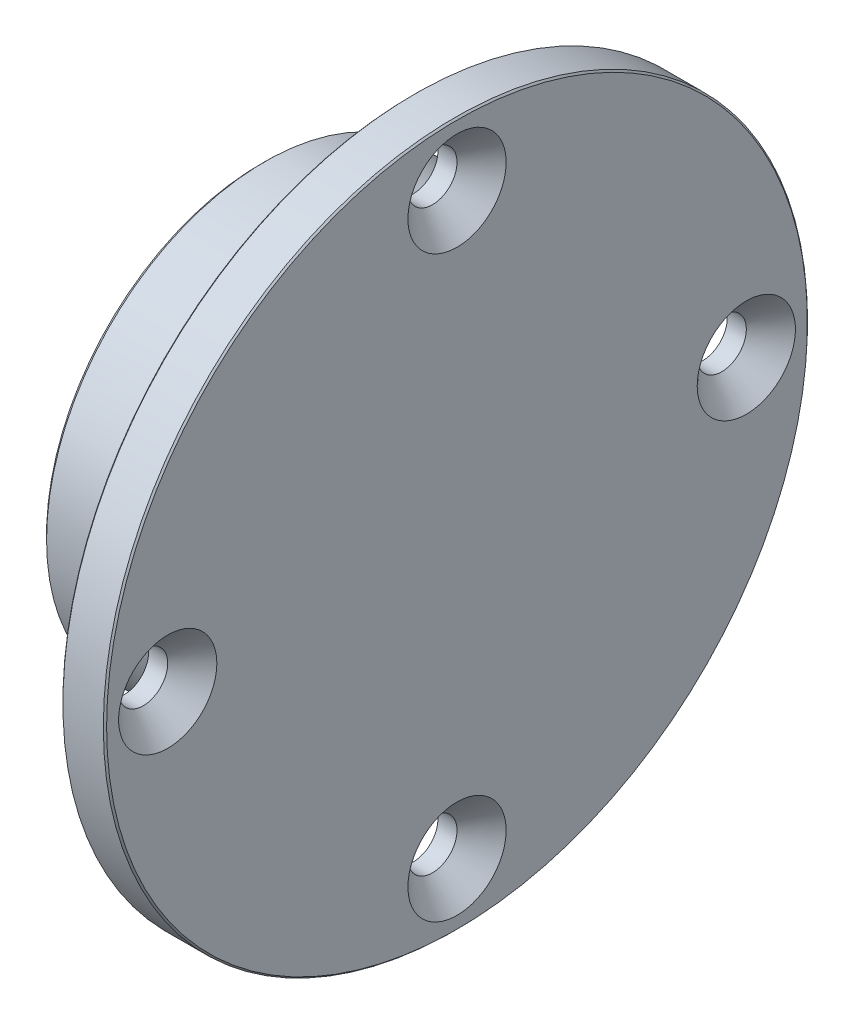
SolidWorks part; units mm, degrees
material "6063-T6"
ref_plane "Front Plane" through (0, 0, 0) normal (0, 0, 1) x (1, 0, 0)
ref_plane "Top Plane" through (0, 0, 0) normal (0, 1, 0) x (1, 0, 0)
ref_plane "Right Plane" through (0, 0, 0) normal (1, 0, 0) x (0, 0, -1)
sketch "Sketch1" plane through (0, 0, 0) normal (0, 0, 1) x (1, 0, 0)
  line L0 (0, 16) -> (1.6954, 16)
  line L1 (13, 16) -> (13, 12.5)
  line L2 (13, 12.5) -> (15, 12.5)
  line L3 (15, 12.5) -> (15, 0)
  line L4 (15, 0) -> (18, 0)
  line L5 (18, 0) -> (18, 32.5)
  line L6 (18, 32.5) -> (14, 32.5)
  line L7 (14, 32.5) -> (14, 20)
  line L8 (14, 20) -> (0, 20)
  line L9 (0, 20) -> (0, 16)
  line L10 (1.6954, 16) -> (1.6954, 16.85)
  line L11 (1.6954, 16.85) -> (2.9954, 16.85)
  line L12 (2.9954, 16.85) -> (2.9954, 16)
  line L13 (2.9954, 16) -> (13, 16)
  dimension "D1" = 16
  dimension "D2" = 2
  dimension "D3" = 12.5
  dimension "D4" = 18
  dimension "D5" = 4
  dimension "D6" = 3
  dimension "D7" = 20
  dimension "D8" = 32.5
  dimension "D9" = 1.3
  dimension "D10" = 16.85
  dimension "D11" = 10.0046
revolve "Revolve1" add sketch "Sketch1" angle 360 about L4
sketch "Sketch2" plane through (0, 0, 0) normal (0, 1, 0) x (1, 0, 0)
  line L0 (14, 26.5) -> (18, 26.5)
  line L1 (14, 32.5) -> (14, -32.5) construction
  line L2 (18, -32.5) -> (18, 32.5) construction
  line L3 (18, 26.5) -> (18, 31)
  line L4 (18, 31) -> (15.75, 28.75)
  line L5 (15.75, 28.75) -> (14, 28.75)
  line L6 (14, 28.75) -> (14, 26.5)
  dimension "D1" = 26.5
  dimension "D2" = 2.25
  dimension "D3" = 4.5
  dimension "D4" = 45
revolve "Cut-Revolve1" cut sketch "Sketch2" angle 360 about L0
pattern_circular "CirPattern1" count 4 over 360 about axis through (0, 0, 0) along (1, 0, 0) of "Cut-Revolve1"
chamfer "Chamfer1" distance 0.4 angle 45 5 edges at (13, 0, 12.5) (0, 0, 16) (18, 0, 32.5) (14, 0, 32.5) (0, 0, 20)
hole_wizard "M4 Tapped Hole1" positions "Sketch4" profile "Sketch5" tap size "M4" standard "GB"
sketch "Sketch4" plane through (18, 0, 0) normal (1, 0, 0) x (0, 0, -1)
  line L0 (0, 0) -> (26.5, 0) construction
  line L2 (0, 0) -> (10.0763, 10.0763) construction
  circle A0 centre (0, 0) radius 14.25
  point P13 (10.0763, 10.0763)
  dimension "D1" = 28.5
  dimension "D2" = 45
cosmetic thread "Hole thread1" [suppressed] parameters "D2"=4
sketch "Sketch5" plane through (18, 10.0763, -10.0763) normal (0, 1, 0) x (0, 0, -1)
  line L0 (0, 0) -> (0, 18)
  line L1 (0, 18) -> (1.65, 18)
  line L2 (1.65, 18) -> (1.65, 0)
  line L5 (1.65, 0) -> (0, 0)
  line L11 (0, -6.35) -> (0, 107.95) construction
  dimension "通孔螺纹孔钻头直径" = 3.3
  dimension "通孔螺纹孔钻头深度" = 18
pattern_circular "CirPattern2" [suppressed] count 2 over 360
sketch "Sketch6" plane through (18, 0, 0) normal (1, 0, 0) x (0, 0, -1)
  circle A0 centre (0, 0) radius 32.25
  circle A1 centre (0, 0) radius 32.5
  dimension "D1" = 64.5
  dimension "D2" = 65
extrude "Cut-Extrude1" cut sketch "Sketch6" against normal blind 10
